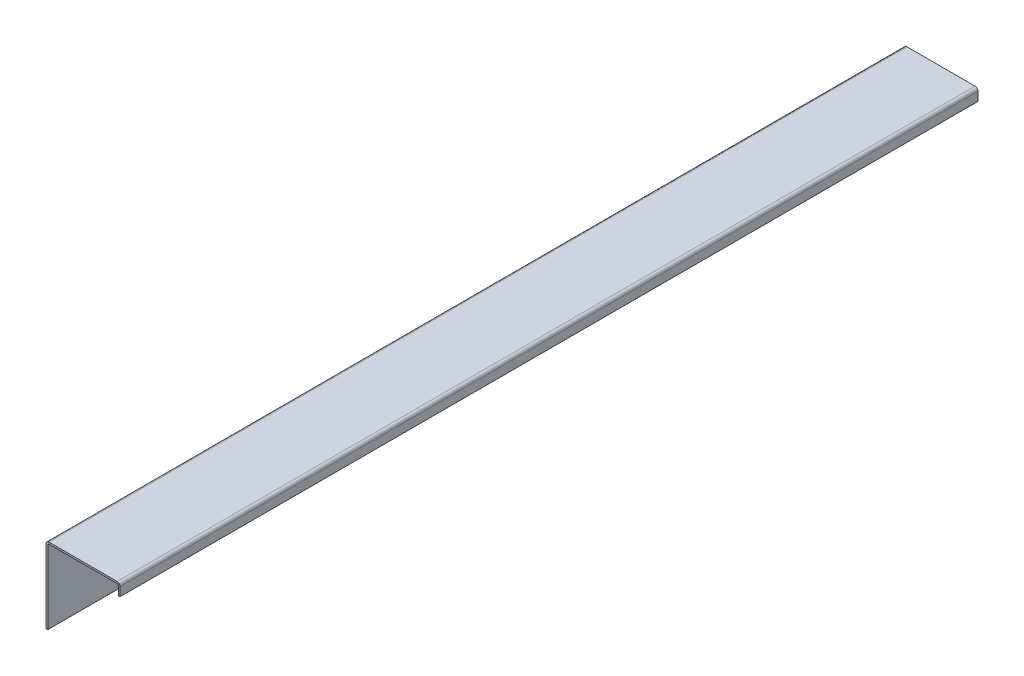
from build123d import *

# Parameters (mm, degrees)
BOSS_EXTRUDE1_DEPTH = 1460
SKETCH2_R           = 4
CUT_EXTRUDE1_DEPTH  = 1460


with BuildPart() as part:
    # Sketch1 → Boss-Extrude1 (new body)
    with BuildSketch(Plane.XY):
        with BuildLine():
            Line((0, 0), (0, 125))
            ThreePointArc((0, 125), (1.464466094, 128.535533906), (5, 130))
            Line((5, 130), (121, 130))
            ThreePointArc((121, 130), (124.535533906, 128.535533906), (126, 125))
            Line((126, 125), (126, 110))
            Line((126, 110), (123, 110))
            Line((123, 110), (123, 125))
            ThreePointArc((123, 125), (122.414213562, 126.414213562), (121, 127))
            Line((121, 127), (5, 127))
            ThreePointArc((5, 127), (3.585786438, 126.414213562), (3, 125))
            Line((3, 125), (3, 0))
            Line((3, 0), (0, 0))
        make_face()
    extrude(amount=BOSS_EXTRUDE1_DEPTH)

    # Sketch2 → Cut-Extrude1 (cut)
    with BuildSketch(Plane.ZY):
        with Locations((121, 80)):
            Circle(SKETCH2_R)
        with Locations((1339, 80)):
            Circle(SKETCH2_R)
        with Locations((933, 80)):
            Circle(SKETCH2_R)
        with Locations((527, 80)):
            Circle(SKETCH2_R)
        with Locations((121, 20)):
            Circle(SKETCH2_R)
        with Locations((1339, 20)):
            Circle(SKETCH2_R)
        with Locations((933, 20)):
            Circle(SKETCH2_R)
        with Locations((527, 20)):
            Circle(SKETCH2_R)
    extrude(amount=-CUT_EXTRUDE1_DEPTH, mode=Mode.SUBTRACT)


solid = part.part
